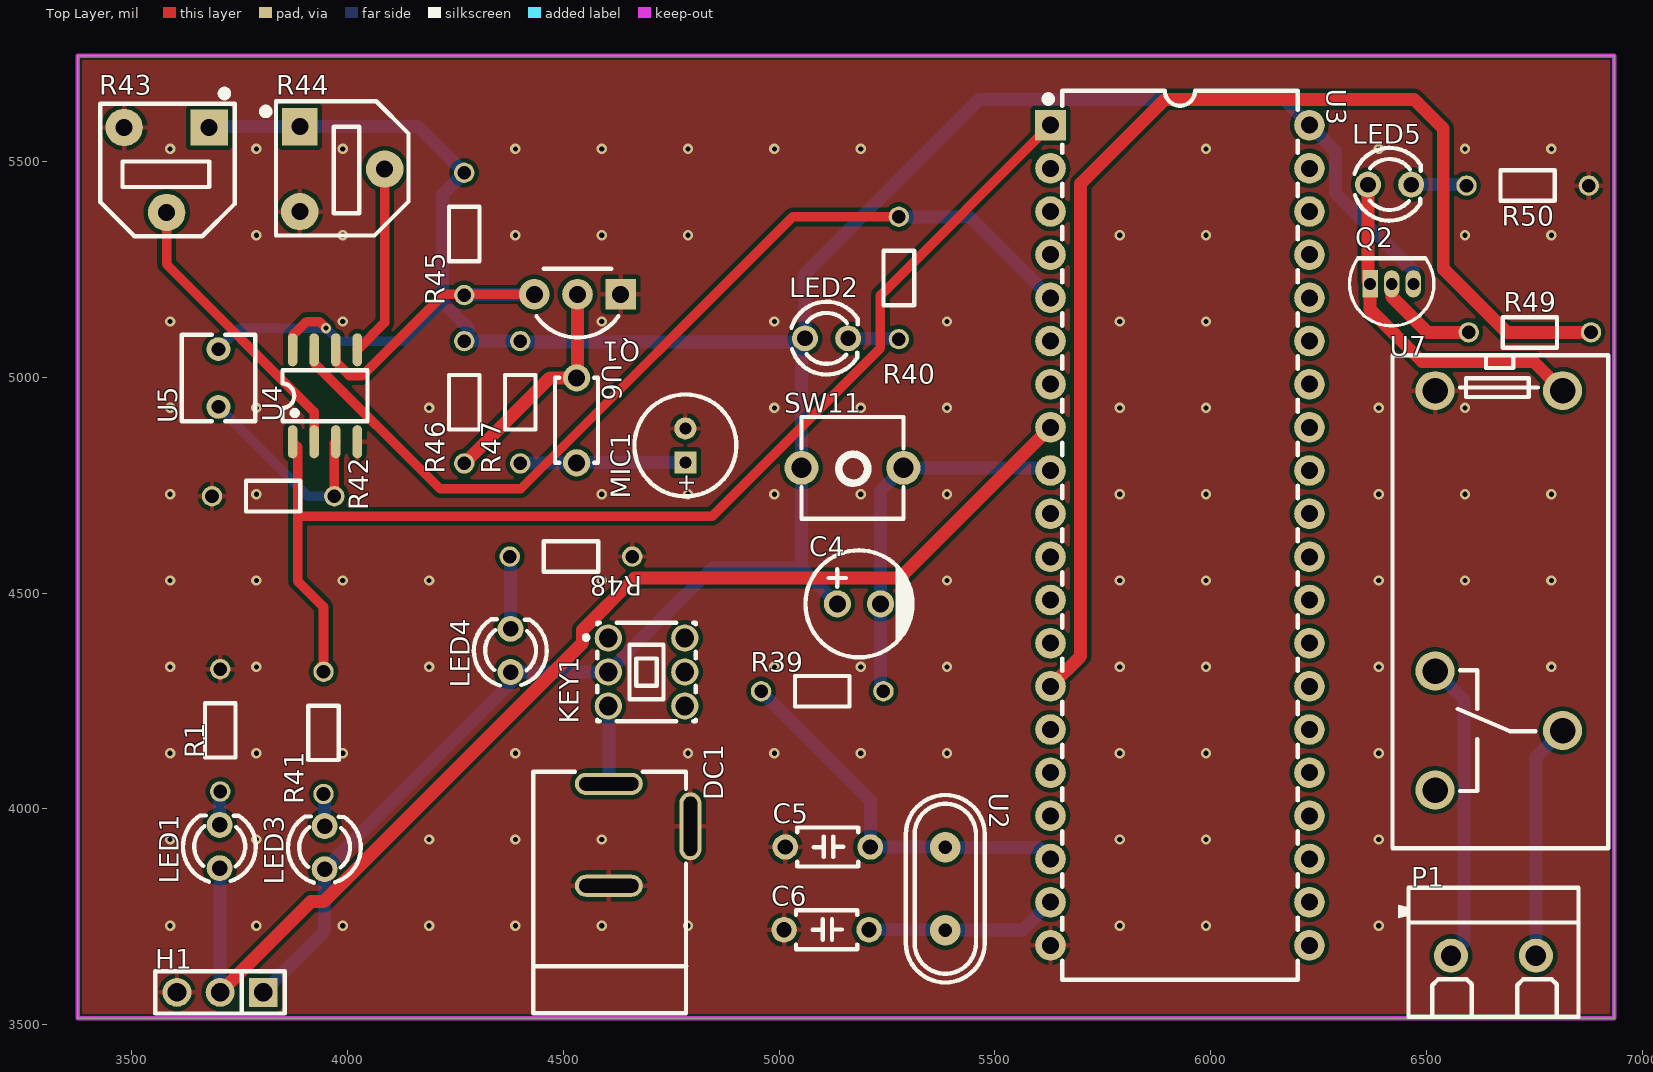
[diagram p0: Top Layer view]
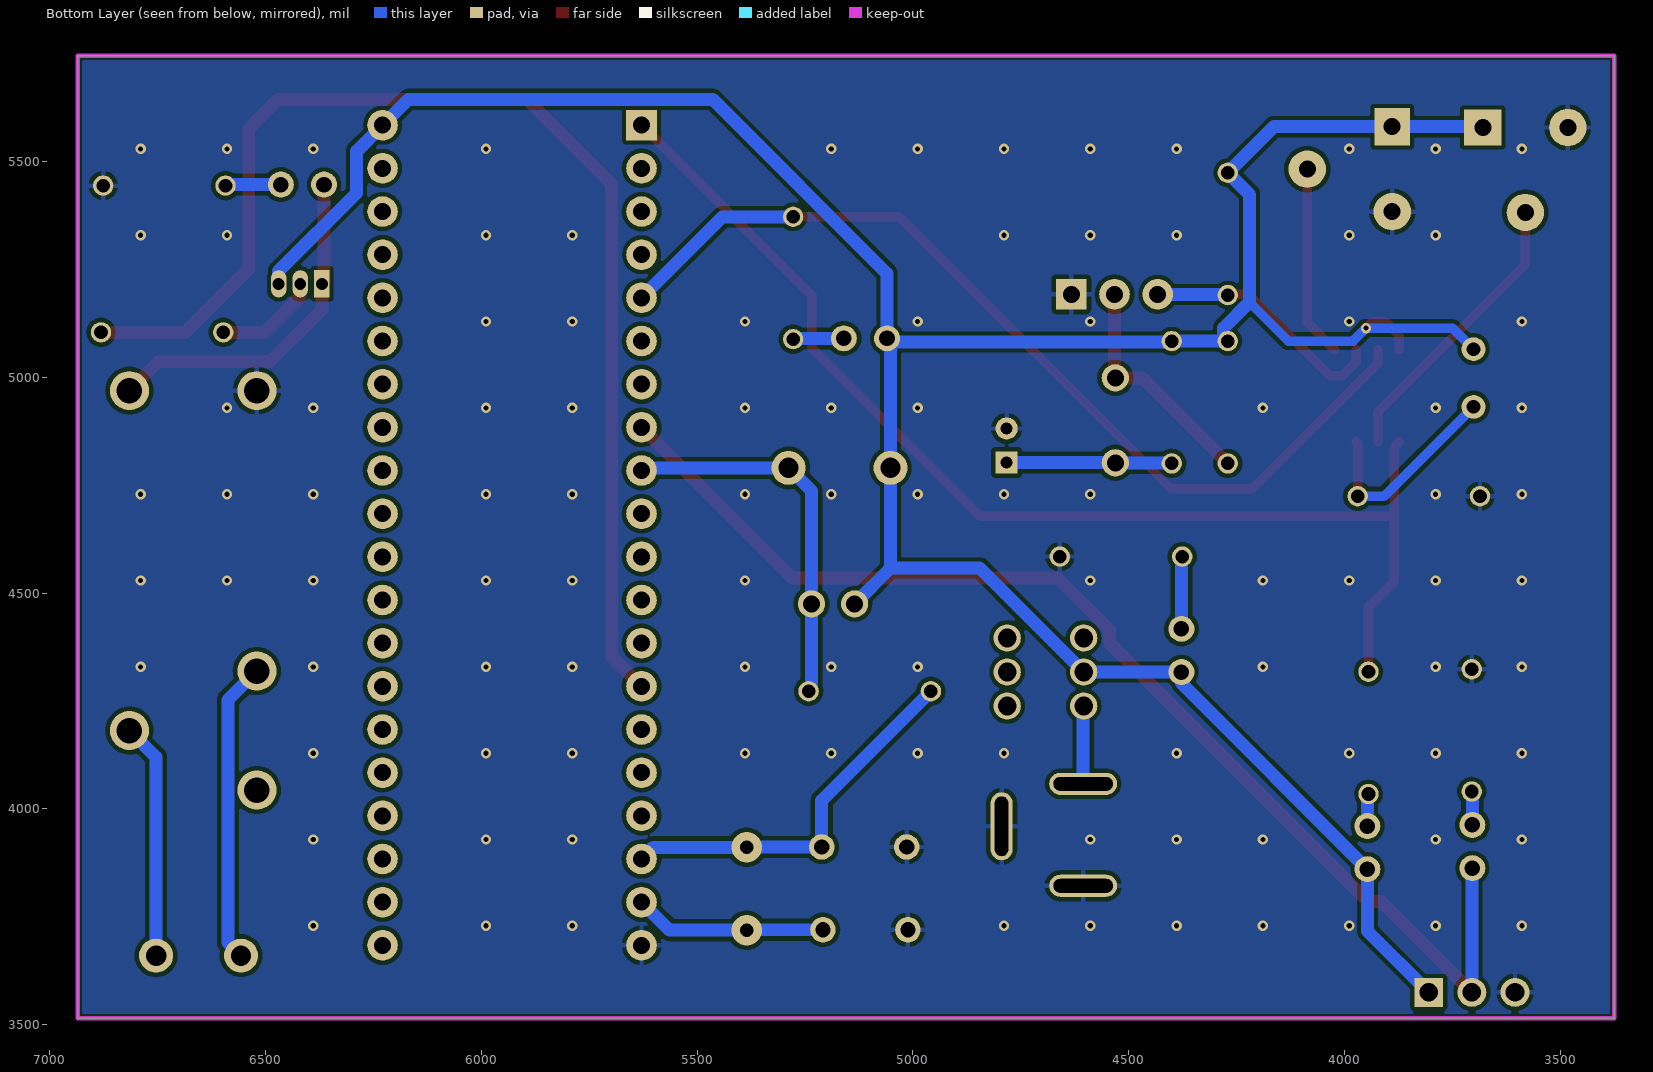
[diagram p1: Bottom Layer view, seen from below]
# Altium PCB MISC75177.pcbdoc
Units mil, origin at the board's own origin, x right, y up, seen from the top; angles counter-clockwise.
Board outline 3560 x 2230 mil, 2 copper layers (Top Layer, Bottom Layer), stack 62.206 mil thick; 35 components, 28 nets, 127 pads, 101 vias.

## Layer stack, top to bottom
Top Solder Mask Layer: solder mask 0.394, Dk 3.3
Top Layer: signal copper 1.379
Dielectric1: surface 59.449, FR4, Dk 4.5
Bottom Layer: signal copper 1.378
Bottom Solder Mask Layer: solder mask 0.394, Dk 3.3

## Board outline
3375,5745 3375,3515 6935,3515 6935,5745

## Design rules (kind name [scope] priority, off if disabled: settings)
BoardOutlineClearance copperThickness2oz_1 [All] p2 off: genericclearance=7.99 ignorepadtopadclearanceinfootprint=FALSE except(0: Arc-SplitContinuation Track-SplitContinuation SMDPad-SplitContinuation THPad-SplitContinuation Via-SplitContinuation Fill-SplitContinuation Region-SplitContinuation Poly-SplitContinuation Text-SplitContinuation Hole-SplitContinuation; 5.98: Arc-CutoutEdge Track-CutoutEdge SMDPad-CutoutEdge THPad-CutoutEdge Via-CutoutEdge Text-CutoutEdge; 6.89: Hole-OutlineEdge Hole-CutoutEdge; 10: Poly-OutlineEdge Poly-CutoutEdge; 11.81: Arc-OutlineEdge Track-OutlineEdge SMDPad-OutlineEdge THPad-OutlineEdge Via-OutlineEdge Fill-OutlineEdge Region-OutlineEdge Text-OutlineEdge Fill-CutoutEdge Region-CutoutEdge)
BoardOutlineClearance Plane_innerPlane_1 [All] p4 off: genericclearance=4.02 ignorepadtopadclearanceinfootprint=FALSE except(0: Arc-SplitContinuation Track-SplitContinuation SMDPad-SplitContinuation THPad-SplitContinuation Via-SplitContinuation Fill-SplitContinuation Region-SplitContinuation Poly-SplitContinuation Text-SplitContinuation Hole-SplitContinuation; 5.98: Arc-CutoutEdge Track-CutoutEdge SMDPad-CutoutEdge THPad-CutoutEdge Via-CutoutEdge Text-CutoutEdge; 6.89: Hole-OutlineEdge Hole-CutoutEdge; 10: Poly-OutlineEdge Poly-CutoutEdge; 11.81: Arc-OutlineEdge Track-OutlineEdge SMDPad-OutlineEdge THPad-OutlineEdge Via-OutlineEdge Fill-OutlineEdge Region-OutlineEdge Text-OutlineEdge Fill-CutoutEdge Region-CutoutEdge)
BoardOutlineClearance Copper_copperRegion_1 [All] p6 off: genericclearance=4.02 ignorepadtopadclearanceinfootprint=FALSE except(0: Arc-SplitContinuation Track-SplitContinuation SMDPad-SplitContinuation THPad-SplitContinuation Via-SplitContinuation Fill-SplitContinuation Region-SplitContinuation Poly-SplitContinuation Text-SplitContinuation Hole-SplitContinuation; 5.98: Arc-CutoutEdge Track-CutoutEdge SMDPad-CutoutEdge THPad-CutoutEdge Via-CutoutEdge Text-CutoutEdge; 6.89: Hole-OutlineEdge Hole-CutoutEdge; 10: Poly-OutlineEdge Poly-CutoutEdge; 11.81: Arc-OutlineEdge Track-OutlineEdge SMDPad-OutlineEdge THPad-OutlineEdge Via-OutlineEdge Fill-OutlineEdge Region-OutlineEdge Text-OutlineEdge Fill-CutoutEdge Region-CutoutEdge)
BoardOutlineClearance copperThickness1oz_1 [All] p8: genericclearance=4.02 ignorepadtopadclearanceinfootprint=FALSE except(0: Arc-SplitContinuation Track-SplitContinuation SMDPad-SplitContinuation THPad-SplitContinuation Via-SplitContinuation Fill-SplitContinuation Region-SplitContinuation Poly-SplitContinuation Text-SplitContinuation Hole-SplitContinuation; 5.98: Arc-CutoutEdge Track-CutoutEdge SMDPad-CutoutEdge THPad-CutoutEdge Via-CutoutEdge Text-CutoutEdge; 6.89: Hole-OutlineEdge Hole-CutoutEdge; 10: Poly-OutlineEdge Poly-CutoutEdge; 11.81: Arc-OutlineEdge Track-OutlineEdge SMDPad-OutlineEdge THPad-OutlineEdge Via-OutlineEdge Fill-OutlineEdge Region-OutlineEdge Text-OutlineEdge Fill-CutoutEdge Region-CutoutEdge)
Clearance copperThickness2oz [All] p1 off: gap=7.99 ignorepadtopadclearanceinfootprint=FALSE except(5.98: SMDPad-Track SMDPad-SMDPad THPad-Track SMDPad-THPad THPad-THPad Track-Via SMDPad-Via THPad-Via Via-Via Fill-SMDPad Region-SMDPad Fill-THPad Region-THPad Fill-Via Region-Via Fill-Fill Fill-Region Region-Region Arc-Track Arc-SMDPad Arc-THPad Arc-Via Fill-Arc Region-Arc Arc-Arc Text-Track SMDPad-Text Text-THPad Text-Via Fill-Text Region-Text Arc-Text Text-Text; 6.89: Hole-Track Hole-SMDPad Hole-THPad Hole-Via Fill-Hole Region-Hole Hole-Arc Hole-Text; 10: Poly-Track Poly-SMDPad Poly-THPad Poly-Via Poly-Fill Poly-Region Poly-Poly Poly-Arc Poly-Text Poly-Hole; 11.81: Fill-Track Region-Track)
Clearance Plane_innerPlane [All] p3 off: gap=4.02 ignorepadtopadclearanceinfootprint=FALSE except(5.98: SMDPad-Track SMDPad-SMDPad THPad-Track SMDPad-THPad THPad-THPad Track-Via SMDPad-Via THPad-Via Via-Via Fill-SMDPad Region-SMDPad Fill-THPad Region-THPad Fill-Via Region-Via Fill-Fill Fill-Region Region-Region Arc-Track Arc-SMDPad Arc-THPad Arc-Via Fill-Arc Region-Arc Arc-Arc Text-Track SMDPad-Text Text-THPad Text-Via Fill-Text Region-Text Arc-Text Text-Text; 6.89: Hole-Track Hole-SMDPad Hole-THPad Hole-Via Fill-Hole Region-Hole Hole-Arc Hole-Text; 10: Poly-Track Poly-SMDPad Poly-THPad Poly-Via Poly-Fill Poly-Region Poly-Poly Poly-Arc Poly-Text Poly-Hole; 11.81: Fill-Track Region-Track)
Clearance Copper_copperRegion [All] p5 off: gap=4.02 ignorepadtopadclearanceinfootprint=FALSE except(5.98: SMDPad-Track SMDPad-SMDPad THPad-Track SMDPad-THPad THPad-THPad Track-Via SMDPad-Via THPad-Via Via-Via Fill-SMDPad Region-SMDPad Fill-THPad Region-THPad Fill-Via Region-Via Fill-Fill Fill-Region Region-Region Arc-Track Arc-SMDPad Arc-THPad Arc-Via Fill-Arc Region-Arc Arc-Arc Text-Track SMDPad-Text Text-THPad Text-Via Fill-Text Region-Text Arc-Text Text-Text; 6.89: Hole-Track Hole-SMDPad Hole-THPad Hole-Via Fill-Hole Region-Hole Hole-Arc Hole-Text; 10: Poly-Track Poly-SMDPad Poly-THPad Poly-Via Poly-Fill Poly-Region Poly-Poly Poly-Arc Poly-Text Poly-Hole; 11.81: Fill-Track Region-Track)
Clearance copperThickness1oz [All] p7: gap=4.02 ignorepadtopadclearanceinfootprint=FALSE except(5.98: SMDPad-Track SMDPad-SMDPad THPad-Track SMDPad-THPad THPad-THPad Track-Via SMDPad-Via THPad-Via Via-Via Fill-SMDPad Region-SMDPad Fill-THPad Region-THPad Fill-Via Region-Via Fill-Fill Fill-Region Region-Region Arc-Track Arc-SMDPad Arc-THPad Arc-Via Fill-Arc Region-Arc Arc-Arc Text-Track SMDPad-Text Text-THPad Text-Via Fill-Text Region-Text Arc-Text Text-Text; 6.89: Hole-Track Hole-SMDPad Hole-THPad Hole-Via Fill-Hole Region-Hole Hole-Arc Hole-Text; 10: Poly-Track Poly-SMDPad Poly-THPad Poly-Via Poly-Fill Poly-Region Poly-Poly Poly-Arc Poly-Text Poly-Hole; 11.81: Fill-Track Region-Track)
DiffPairsRouting differentialPair [All] p1: maxlimit=6 minlimit=6 mostfreqgap=6 toplayer_minwidth=5 toplayer_prefwidth=10 toplayer_maxwidth=100 toplayer_mingap=6 toplayer_prefgap=6 toplayer_maxgap=6 bottomlayer_minwidth=5 bottomlayer_prefwidth=10 bottomlayer_maxwidth=100 bottomlayer_mingap=6 bottomlayer_prefgap=6 bottomlayer_maxgap=6 maxuncoupledlength=10
HoleToHoleClearance otherClearance [All] p1: gap=11.81 allowstackedmicrovias=TRUE
Length netLength [All] p1: minlimit=0 maxlimit=0
PasteMaskExpansion pasteMaskExpansion [All] p1: expansion=0
PlaneConnect innerPlane [All] p1: planeconnectstyle=Relief reliefexpansion=20 reliefentries=4 reliefconductorwidth=10 reliefairgap=10
PolygonConnect copperRegion [All] p1: connectstyle=Relief reliefconductorwidth=10 reliefentries=4 polygonreliefangle="90 Angle" airgapwidth=10 via.connectstyle=Relief via.reliefconductorwidth=10 via.reliefentries=4 via.polygonreliefangle="90 Angle" via.airgapwidth=10
RoutingVias viaSize [All] p1: holewidth=12.01 width=24.02 viastyle="Through Hole" minholewidth=11.81 minwidth=19.68 maxholewidth=248.03 maxwidth=393.7
SolderMaskExpansion solderMaskExpansion [IsVia] p1: expansion=-1000 istentingtop=TRUE
SolderMaskExpansion solderMaskExpansion [All] p2: expansion=2.01 istentingtop=FALSE
Width copperThickness2oz_2 [All] p1 off: maxlimit=100 minlimit=8 preferedwidth=10
Width copperThickness1oz_2 [All] p2: maxlimit=100 minlimit=5 preferedwidth=30

## Components (designator, comment, footprint, x,y, rotation, side; value= is the part's Value field where it differs from the comment)
C4 "10uF" CAP-TH_BD6.3-P2.50-D1.0-FD 5185,4475 r0 top
C5 "30pF" CAP-TH_L3.6-W2.3-P5.00-D0.5 5112.86,3911.76 r0 top
C6 "30pF" CAP-TH_L3.6-W2.3-P5.00-D0.5 5110,3720 r0 top
DC1 "" DC-2.0 4595,3935 r270 top
H1 "" HDR-TH_3P-P2.54-V-M 3705,3575 r180 top
KEY1 "Self-locking switch 5.8Z white-grey-white 260G" SW-TH_6P-L5.8-W5.8-P2.00-LS4.5-TR 4692.91,4317.05 r90 top
LED1 "" LED_TH-3mm 3703.98,3912.73 r90 top
LED2 "" LED_TH-3mm 5110,5090 r0 top
LED3 "" LED_TH-3mm 3947.07,3910.3 r90 top
LED4 "" LED_TH-3mm 4377.91,4367.05 r90 top
LED5 "" LED_TH-3mm 6414.31,5446.49 r0 top
MIC1 "MIC" MIC-TH_BD6.0-P2.00 4782.91,4842.05 r90 top
P1 "KF301-2P terminal block" CONN-TH_XY301V-A-5.0-2P 6655,3660 r180 top
Q1 "9014" TO-92-3_L4.9-W3.7-P2.54-L 4532.91,5192.05 r180 top
Q2 "9012-H" TO-92-3_L4.9-W3.7-P1.27-R 6419.31,5216.49 r180 top
R1 "2kΩ" Res_1/8W 3702.91,4182.05 r270 top
R39 "10kΩ" Res_1/8W 5100,4270 r0 top
R40 "2kΩ" Res_1/8W 5275,5230 r270 top
R41 "2kΩ" Res_1/8W 3947.07,4176.25 r90 top
R42 "2kΩ" Res_1/8W 3827.91,4722.05 r0 top
R43 "10kΩ" RES-ADJ-SMD_RM065-V1 3581.16,5480.22 r180 top
R44 "10kΩ" RES-ADJ-SMD_RM065-V1 3987.91,5482.05 r270 top
R45 "20kΩ" Res_1/8W 4272.91,5332.05 r90 top
R46 "2.2MΩ" Res_1/8W 4272.91,4942.05 r90 top
R47 "10kΩ" Res_1/8W 4402.91,4942.05 r90 top
R48 "2kΩ" Res_1/8W 4517.91,4587.05 r180 top
R49 "2kΩ" Res_1/8W 6739.31,5101.49 r0 top
R50 "2kΩ" Res_1/8W 6734.31,5446.49 r180 top
SW11 "Tact switch, 6*6*5 plastic head, 260G, travel 0.25mm, through-hole, middle 2 pins" KEY-TH_2P-L6.0-W6.0-P5.00 5170,4790 r0 top
U2 "12MHz" HC-49US_L11.0-W4.6-P4.88 5385,3815 r270 top
U3 "STC89C516RD+40I-PDIP40" DIP-40_L52.3-W13.9-P2.54-LS15.2-BL 5928.71,4633.94 r270 top
U4 "LM393DR2G" SOIC-8_L5.0-W4.0-P1.27-LS6.0-BL 3947.91,4957.05 r0 top
U5 "光敏电阻-5MM" RES-TH_L4.9-W4.3-P3.4 3701.16,4998.21 r90 top
U6 "100nF" CAP-TH_L5.0-W2.5-P5.00-D1.0 4531.03,4900.22 r270 top
U7 "SSKD6132" RELAY-TH_G2R-1 6667.51,4506.34 r270 top

## Footprints (in the part's own frame and the unit in brackets; to place one, negate y for a bottom-side part, rotate by r counter-clockwise, add the part's x,y. Pads: shape width x height; smd on the part's side, far side on the other; paste and mask are expansions set on the pad)
CAP-TH_BD6.3-P2.50-D1.0-FD [mm]
  round 1.6 hole 1: 1(-1.27,0) 2(1.27,0)
  silkscreen extent -3.15,-3.15 3.17,3.15
CAP-TH_L3.6-W2.3-P5.00-D0.5 [mm]
  round 1.5 hole 0.9: 1(-2.5,0) 2(2.5,0)
  silkscreen extent -1.8,-1.15 1.8,1.15
CAP-TH_L5.0-W2.5-P5.00-D1.0 [mm]
  round 1.6 hole 1: 1(-2.5,0) 2(2.5,0)
  silkscreen extent -2.5,-1.27 2.5,1.25
CONN-TH_XY301V-A-5.0-2P [mm]
  round 2 hole 1.2: 1(-2.5,0) 2(2.5,0)
  silkscreen extent -5,-4 5.6,3.6
DC-2.0 [mil]
  oval 157.5x51.2 hole 31.5 slot 137.8 at 0 deg paste+0 mask+2: 2(-24.7,199.5)
  oval 51.2x157.5 hole 31.5 slot 137.8 at 90 deg paste+0 mask+2: 3(113.1,10.5) 4(-123.1,10.5)
  silkscreen extent -151,-165 408,190
DIP-40_L52.3-W13.9-P2.54-LS15.2-BL [mm]
  rect 1.8x1.8 hole 1: 1(-24.13,-7.62)
  round 1.8 hole 1: 2(-21.59,-7.62) 3(-19.05,-7.62) 4(-16.51,-7.62) 5(-13.97,-7.62) 6(-11.43,-7.62) 7(-8.89,-7.62) 8(-6.35,-7.62) 9(-3.81,-7.62) 10(-1.27,-7.62) 11(1.27,-7.62) 12(3.81,-7.62) 13(6.35,-7.62) 14(8.89,-7.62) 15(11.43,-7.62) 16(13.97,-7.62) 17(16.51,-7.62) 18(19.05,-7.62) 19(21.59,-7.62) 20(24.13,-7.62) 21(24.13,7.62) 22(21.59,7.62) 23(19.05,7.62) 24(16.51,7.62) 25(13.97,7.62) 26(11.43,7.62) 27(8.89,7.62) 28(6.35,7.62) 29(3.81,7.62) 30(1.27,7.62) 31(-1.27,7.62) 32(-3.81,7.62) 33(-6.35,7.62) 34(-8.89,7.62) 35(-11.43,7.62) 36(-13.97,7.62) 37(-16.51,7.62) 38(-19.05,7.62) 39(-21.59,7.62) 40(-24.13,7.62)
  silkscreen extent -26.16,-7.95 26.16,6.93
HC-49US_L11.0-W4.6-P4.88 [mm]
  round 1.8 hole 0.8: 1(-2.44,0) 2(2.44,0)
  silkscreen extent -5.51,-2.32 5.51,2.32
HDR-TH_3P-P2.54-V-M [mm]
  rect 1.7x1.7 hole 1.1: 1(-2.54,0)
  round 1.7 hole 1.1: 2(0,0) 3(2.54,0)
  silkscreen extent -3.81,-1.25 3.81,1.25
KEY-TH_2P-L6.0-W6.0-P5.00 [mm]
  round 2 hole 1.2: 1(-3,0) 2(3,0)
  silkscreen extent -3,-3 3,3
LED_TH-3mm [mil]
  round 60 hole 36 paste+0 mask+2: 1(-50,0) 2(50,0)
  silkscreen extent -81,-84 72,85
MIC-TH_BD6.0-P2.00 [mm]
  rect 1.3x1.3 hole 0.7: 1(-1,0)
  round 1.3 hole 0.7: 2(1,0)
  silkscreen extent -3,-3 3,3
RELAY-TH_G2R-1 [mm]
  round 2.3 hole 1.5: 1(-11.75,-3.75) 2(4.75,-3.75) 3(11.75,-3.75) 4(8.25,3.75) 5(-11.75,3.75)
  silkscreen extent -13.83,-6.26 15.17,6.44
RES-ADJ-SMD_RM065-V1 [mm]
  rect 2.2x2.1 hole 1 paste+0 mask+0.05: 1(-2.5,-2.5)
  round 2.2 hole 1 paste+0 mask+0.05: 2(0,2.5) 3(2.5,-2.5)
  silkscreen extent -4,-4.7 3.9,3.9
RES-TH_L4.9-W4.3-P3.4 [mm]
  round 1.4 hole 0.8 paste+0 mask+0.05: 1(-1.7,0) 2(1.7,0)
  silkscreen extent -2.54,-2.16 2.54,2.16
Res_1/8W [mil]
  round 47.2 hole 31.5 paste+0 mask+2: 1(-141.7,2.48) 2(141.7,2.48)
  silkscreen extent -63,-33 63,38
SOIC-8_L5.0-W4.0-P1.27-LS6.0-BL [mil]
  oval 22.38x76.78 smd: 1(-75,-106.5) 2(-25,-106.5) 3(25,-106.5) 4(75,-106.5) 5(75,106.5) 6(25,106.5) 7(-25,106.5) 8(-75,106.5)
  silkscreen extent -98,-59 98,59
SW-TH_6P-L5.8-W5.8-P2.00-LS4.5-TR [mm]
  round 1.6 hole 1.1: 1(2,2.25) 2(0,2.25) 3(-2,2.25) 4(-2,-2.25) 5(0,-2.25) 6(2,-2.25)
  silkscreen extent -2.9,-2.9 2.9,3.68
TO-92-3_L4.9-W3.7-P1.27-R [mm]
  rect 0.9x1.6 hole 0.7: 1(1.27,0)
  oval 0.9x1.6 hole 0.7: 2(0,0) 3(-1.27,0)
  silkscreen extent -2.48,-1.5 2.48,2.48
TO-92-3_L4.9-W3.7-P2.54-L [mm]
  rect 1.8x1.8 hole 1: 1(-2.54,0)
  round 1.8 hole 1: 2(0,0) 3(2.54,0)
  silkscreen extent -2.41,-1.5 2.41,2.54

## Via types
v1: diameter 24.02, hole 12, Top Layer to Bottom Layer, 101 vias

## Nets (pads, with @x,y where several pads share a name; then routed paths per layer and width w, separated by ;. In a path a pad name is that pad's centre, name@x,y a point inside that pad or via, vN(x,y) a via of type N, cw(c..) or ccw(c..) an arc to the next point about the centre after c; other vN are vias at no path point)
$1N147: H1.2 LED1.1 U3.8 | length 2771.6
  Top Layer w30: H1.2 3915,3785 3945,3785 4545,4385 4545,4415 4665,4535 5279.77,4535 U3.8
  Bottom Layer w30: LED1.1 3705,3861.71 H1.2
$1N220: LED1.2 R1.2 | length 78.2
  Bottom Layer w30: LED1.2 3703.98,4038.93 R1.2
$1N1459: C5.2 R39.1 U2.1 U3.18 | length 894.5
  Bottom Layer w30: R39.1 5211.29,4019.49 C5.2 5384.3,3911.76 U2.1 5601.59,3911.06 U3.18
$1N1460: C6.2 U2.2 U3.19 | length 447.6
  Bottom Layer w30: C6.2 5383.94,3720 U2.2 5563.71,3718.94 U3.19
$1N1463: C4.2 R39.2 SW11.2 U3.9 | length 885.4
  Bottom Layer w30: R39.2 5235,4279.18 C4.2 5235,4736.89 SW11.2 5622.65,4790 U3.9
$1N1697: LED2.2 R40.2 | length 118.2
  Bottom Layer w30: LED2.2 5275.78,5090 R40.2
$1N1725: R40.1 U3.5 U4.7 | length 2195.4
  Top Layer w22.38: U4.7 3922.91,5033.55 4214.76,4741.7 4401.46,4741.7 5031.46,5371.7 R40.1
  Bottom Layer w30: R40.1 5440.95,5371.7 U3.5
$1N1853: LED3.2 R41.1 | length 75.3
  Bottom Layer w30: R41.1 3947.07,4032.07 LED3.2
$1N2113: R42.2 U4.3 U5.1 | length 481.5
  Top Layer w22.38: R42.2 3969.61,4847.25 U4.3
  Bottom Layer w22.38: U5.1 3907.91,4724.53 R42.2
$1N2302: R43.2 U4.2 | length 672.8
  Top Layer w22.38: R43.2 3581.16,5261.8 3922.91,4920.04 U4.2
$1N2433: R44.2 U4.5 | length 444.8
  Top Layer w22.38: U4.5 4086.34,5126.97 R44.2
$1N2522: Q1.3 R45.1 U4.6 | length 742.8
  Top Layer w22.38: U4.6 3972.91,5035.05 4004.41,5003.55 4034.41,5003.55 4222.91,5192.05 Q1.3
  Bottom Layer w30: R45.1 4272.14,5192.05 Q1.3
$1N2749: Q1.2 R46.1 U6.1 | length 536.9
  Top Layer w30: R46.1 4468.74,4998.65 4531.03,4998.65 4532.91,5000.54 Q1.2
$1N2932: MIC1.1 R47.1 U6.2 | length 383.4
  Bottom Layer w30: R47.1 4401.89,4801.8 U6.2 4531.91,4802.68 MIC1.1
$1N3128: LED4.2 R48.2 | length 168.2
  Bottom Layer w30: R48.2 4377.91,4582.87 LED4.2
$1N3370: DC1.4 KEY1.3 | length 180.7
  Bottom Layer w30: KEY1.3 4605.5,4237.14 DC1.4
$1N3499: P1.1 U7.4 | length 547.1
  Bottom Layer w30: P1.1 6753.43,4119.8 U7.4
$1N3504: P1.2 U7.2 | length 699.4
  Bottom Layer w30: U7.2 6586.57,4252.62 6586.57,3690 P1.2
$1N3587: LED5.1 Q2.1 U7.5 | length 815.6
  Top Layer w30: LED5.1 6364.31,5221.49 Q2.1 6369.31,5156.49 6489.31,5036.49 6747.61,5036.49 U7.5
$1N3733: Q2.2 R49.1 | length 242.5
  Top Layer w30: Q2.2 6419.31,5186.49 6501.83,5103.96 R49.1
$1N3761: R49.2 U3.14 | length 2871
  Top Layer w30: U3.14 5698.74,4353.96 5698.74,5448.74 5893.96,5643.96 6471.04,5643.96 6538.74,5576.26 6538.74,5251.26 6686.04,5103.96 R49.2
$1N3896: LED5.2 R50.2 | length 129.3
  Bottom Layer w30: LED5.2 6590.13,5446.49 R50.2
GND: C5.1 C6.1 DC1.2 DC1.3 H1.3 MIC1.2 Q1.1 R1.1 R42.1 R43.3 R44.3 R48.1 R50.1 U3.20 U4.4 U7.1
  other v1: 3589.1,3729.1 3789.1,3729.1 3989.1,3729.1 4189.1,3729.1 4389.1,3729.1 4589.1,3729.1 4789.1,3729.1 5789.1,3729.1 5989.1,3729.1 6389.1,3729.1 3589.1,3929.1 3789.1,3929.1 4189.1,3929.1 4389.1,3929.1 4589.1,3929.1 5789.1,3929.1 5989.1,3929.1 6389.1,3929.1 3589.1,4129.1 3789.1,4129.1 3989.1,4129.1 4389.1,4129.1 4789.1,4129.1 4989.1,4129.1 5189.1,4129.1 5389.1,4129.1 5789.1,4129.1 5989.1,4129.1 6389.1,4129.1 3589.1,4329.1 3789.1,4329.1 4189.1,4329.1 4989.1,4329.1 5189.1,4329.1 5389.1,4329.1 5789.1,4329.1 5989.1,4329.1 6389.1,4329.1 6789.1,4329.1 3589.1,4529.1 3789.1,4529.1 3989.1,4529.1 4189.1,4529.1 4589.1,4529.1 5389.1,4529.1 5789.1,4529.1 5989.1,4529.1 6389.1,4529.1 6589.1,4529.1 6789.1,4529.1 3589.1,4729.1 3789.1,4729.1 4589.1,4729.1 4789.1,4729.1 4989.1,4729.1 5189.1,4729.1 5389.1,4729.1 5789.1,4729.1 5989.1,4729.1 6389.1,4729.1 6589.1,4729.1 6789.1,4729.1 3589.1,4929.1 3789.1,4929.1 4189.1,4929.1 4989.1,4929.1 5189.1,4929.1 5389.1,4929.1 5789.1,4929.1 5989.1,4929.1 6389.1,4929.1 6589.1,4929.1 3589.1,5129.1 3989.1,5129.1 4589.1,5129.1 4989.1,5129.1 5389.1,5129.1 5789.1,5129.1 5989.1,5129.1 3789.1,5329.1 3989.1,5329.1 4389.1,5329.1 4589.1,5329.1 4789.1,5329.1 5789.1,5329.1 5989.1,5329.1 6589.1,5329.1 6789.1,5329.1 3589.1,5529.1 3789.1,5529.1 3989.1,5529.1 4389.1,5529.1 4589.1,5529.1 4789.1,5529.1 4989.1,5529.1 5189.1,5529.1 5989.1,5529.1 6389.1,5529.1 6589.1,5529.1 6789.1,5529.1
P10: R41.2 U3.1 U4.1 | length 2753.1
  Top Layer w22.38: U4.1 3884.59,4838.87 3884.59,4677.95 ; R41.2 3944.59,4467.95 3884.59,4527.95 3884.59,4677.95 ; U3.1 5234.59,5189.82 5234.59,5067.95 4844.59,4677.95 3884.59,4677.95
P11: U3.2
P12: U3.3
P13: U3.4
VCC: C4.1 H1.1 KEY1.2 LED2.1 LED3.1 LED4.1 Q2.3 R43.1 R44.1 R45.2 R46.2 R47.2 SW11.1 U3.40 U4.8 U5.2 | length 6956.6
  Top Layer w22.38: U4.8 3872.91,5096.23 3905.44,5128.75 3935.44,5128.75 v1(3950.44,5113.75)
  Bottom Layer w22.38: U5.2 3749.77,5113.75 v1(3950.44,5113.75) 3980.44,5083.75 4130.44,5083.75 4220.44,5173.75
  Bottom Layer w30: R43.1 3681.41,5580.47 R44.1 4163.71,5580.47 R45.2 4220.44,5423.75 4220.44,5173.75 4280.44,5113.75 R46.2@4280.44,5083.75 ; H1.1 3947.07,3717.07 LED3.1 4377.91,4291.14 LED4.1 4604.33,4317.05 4845.4,4558.11 5051.89,4558.11 ; R46.2 R46.2@4280.44,5083.75 ; C4.1 5051.89,4558.11 ; Q2.3 6469.31,5246.49 6288.71,5427.08 6288.71,5523.94 U3.40 6168.71,5643.94 5463.94,5643.94 5060,5240 LED2.1 LED2.1@5051.89,5081.89 ; R46.2@4280.44,5083.75 R47.2 4402.3,5081.89 LED2.1@5051.89,5081.89 ; 5051.89,4558.11 SW11.1 LED2.1@5051.89,5081.89
pads on no net: KEY1.1 KEY1.4 KEY1.5 KEY1.6 U3.6 U3.7 U3.10 U3.11 U3.12 U3.13 U3.15 U3.16 U3.17 U3.21 U3.22 U3.23 U3.24 U3.25 U3.26 U3.27 U3.28 U3.29 U3.30 U3.31 U3.32 U3.33 U3.34 U3.35 U3.36 U3.37 U3.38 U3.39 U7.3

## Polygon pours and split planes (outlines as drawn)
GND on Top Layer (solid, remove dead copper, pour order 0): 3000,6005 3000,3335 7180,3335 7180,6005
GND on Bottom Layer (solid, remove dead copper, pour order 2): 3065,5965 3065,3000 7110,3000 7110,5965

## Keep-outs
Board Outline Layer:
  the board outline again, w10